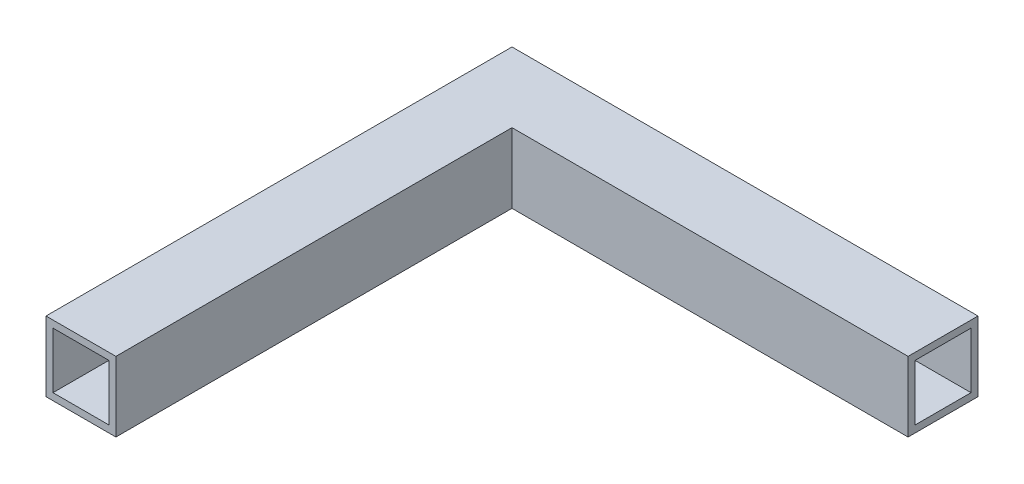
SolidWorks part; units mm, degrees
ref_plane "前视基准面" through (0, 0, 0) normal (0, 0, 1) x (1, 0, 0)
ref_plane "上视基准面" through (0, 0, 0) normal (0, 1, 0) x (1, 0, 0)
ref_plane "右视基准面" through (0, 0, 0) normal (1, 0, 0) x (0, 0, -1)
sketch "草图1" plane through (0, 0, 0) normal (0, 0, 1) x (1, 0, 0)
  line L0 (0, 0) -> (0, 30)
  line L1 (0, 30) -> (200, 30)
  line L2 (200, 30) -> (200, 0)
  line L3 (200, 0) -> (0, 0)
extrude "凸台-拉伸1" add sketch "草图1" against normal blind 30
sketch "草图2" plane through (0, 0, 0) normal (0, 0, 1) x (1, 0, 0)
  line L0 (0, 30) -> (30, 30)
  line L1 (200, 30) -> (0, 30) construction
  line L2 (30, 30) -> (30, 0)
  line L3 (0, 0) -> (200, 0) construction
  line L4 (30, 0) -> (0, 0)
  line L5 (0, 0) -> (0, 30)
extrude "凸台-拉伸2" add sketch "草图2" along normal blind 170
shell "抽壳1" thickness 3
